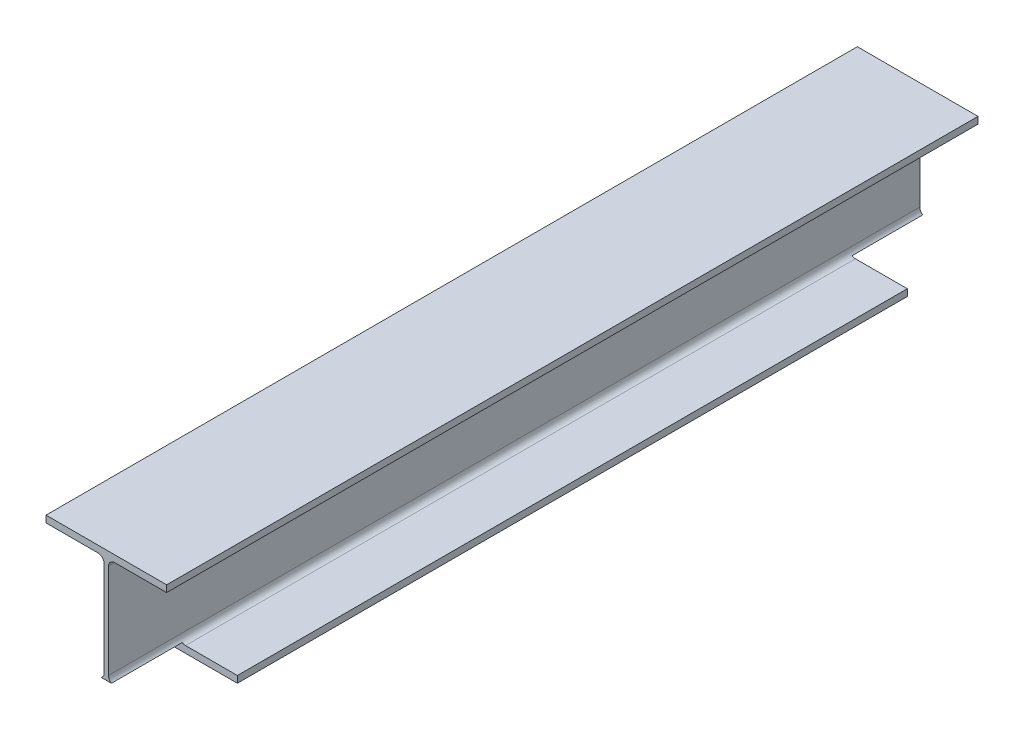
from build123d import *

# Parameters (mm, degrees)
BOSS_EXTRUDE1_DEPTH = 1681
SKETCH3_W           = 250
SKETCH3_H           = 146.5
CUT_EXTRUDE1_DEPTH  = 16


with BuildPart() as part:
    # Sketch1 → Boss-Extrude1 (new body)
    with BuildSketch(Plane.XY):
        with BuildLine():
            Line((0, 0), (250, 0))
            Line((250, 0), (250, 14))
            Line((250, 14), (142.5, 14))
            ThreePointArc((142.5, 14), (133.307611845, 17.807611845), (129.5, 27))
            Line((129.5, 27), (129.5, 223))
            ThreePointArc((129.5, 223), (133.307611845, 232.192388155), (142.5, 236))
            Line((142.5, 236), (250, 236))
            Line((250, 236), (250, 250))
            Line((250, 250), (0, 250))
            Line((0, 250), (0, 236))
            Line((0, 236), (107.5, 236))
            ThreePointArc((107.5, 236), (116.692388155, 232.192388155), (120.5, 223))
            Line((120.5, 223), (120.5, 27))
            ThreePointArc((120.5, 27), (116.692388155, 17.807611845), (107.5, 14))
            Line((107.5, 14), (0, 14))
            Line((0, 14), (0, 0))
        make_face()
    extrude(amount=BOSS_EXTRUDE1_DEPTH)

    # Sketch3 → Cut-Extrude1 (cut)
    with BuildSketch(Plane(origin=(0, 0, 0), x_dir=(-1, 0, 0), z_dir=(0, -1, 0))):
        with Locations((-125, -73.25)):
            Rectangle(SKETCH3_W, SKETCH3_H)
        with Locations((-125, -1607.75)):
            Rectangle(SKETCH3_W, SKETCH3_H)
    extrude(amount=-CUT_EXTRUDE1_DEPTH, mode=Mode.SUBTRACT)


solid = part.part
